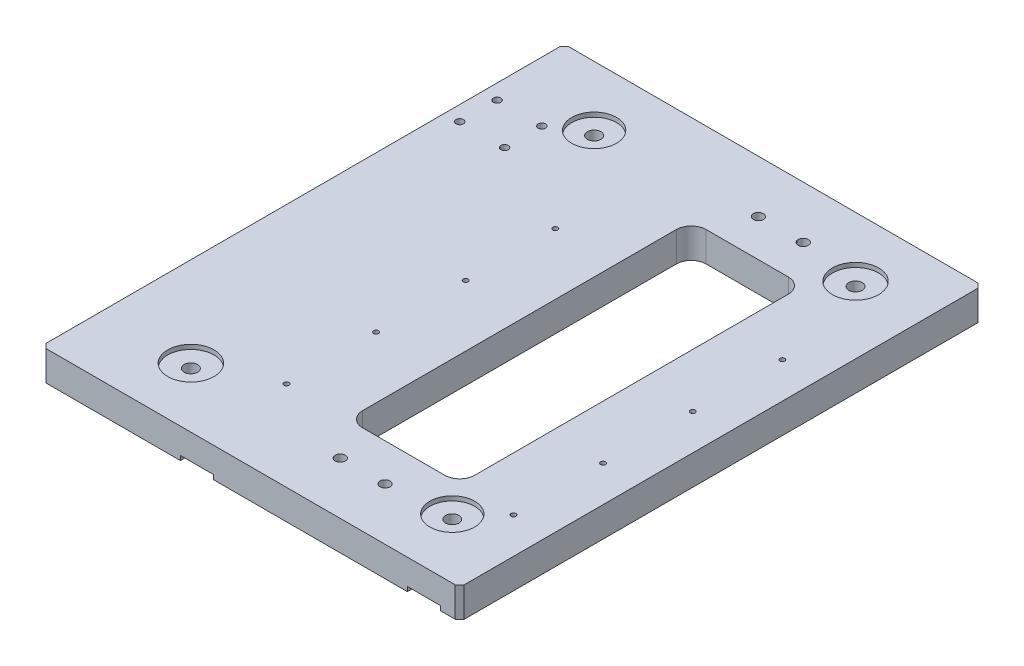
SolidWorks part; units mm, degrees
material "Q235-A"
ref_plane "Front Plane" through (0, 0, 0) normal (0, 0, 1) x (1, 0, 0)
ref_plane "Top Plane" through (0, 0, 0) normal (0, 1, 0) x (1, 0, 0)
ref_plane "Right Plane" through (0, 0, 0) normal (1, 0, 0) x (0, 0, -1)
sketch "Sketch1" plane through (0, 0, 0) normal (0, 0, 1) x (1, 0, 0)
  line L0 (16.7519, 37.3815) -> (146.7519, 37.3815)
  line L1 (-98.2481, 57.3815) -> (181.7519, 57.3815)
  line L2 (-98.2481, 57.3815) -> (-98.2481, 37.3815)
  line L3 (-98.2481, 37.3815) -> (-5.2481, 37.3815)
  line L4 (181.7519, 57.3815) -> (181.7519, 37.3815)
  line L6 (-5.2481, 37.3815) -> (-5.2481, 40.3815)
  line L7 (-5.2481, 40.3815) -> (16.7519, 40.3815)
  line L8 (16.7519, 37.3815) -> (16.7519, 40.3815)
  line L10 (146.7519, 37.3815) -> (146.7519, 40.3815)
  line L11 (146.7519, 40.3815) -> (168.7519, 40.3815)
  line L12 (168.7519, 37.3815) -> (168.7519, 40.3815)
  line L13 (168.7519, 37.3815) -> (181.7519, 37.3815)
  dimension "D1" = 280
  dimension "D2" = 20
  dimension "D3" = 3
  dimension "D4" = 3
  dimension "D5" = 22
  dimension "D6" = 22
  dimension "D7" = 130
  dimension "D8" = 35
extrude "Boss-Extrude1" add sketch "Sketch1" along normal blind 350
chamfer "Chamfer1" distance 3 angle 45 4 edges at (-98.2481, 47.3815, 0) (181.7519, 47.3815, 0) (181.7519, 47.3815, 350) (-98.2481, 47.3815, 350)
sketch "Sketch2" plane through (0, 37.3815, 0) normal (0, -1, 0) x (1, 0, 0)
  line L0 (181.7519, 347) -> (181.7519, 3) construction
  line L1 (46.7519, 290) -> (121.7519, 290)
  line L2 (46.7519, 290) -> (46.7519, 60)
  line L3 (46.7519, 60) -> (121.7519, 60)
  line L4 (121.7519, 290) -> (121.7519, 60)
  line L5 (16.7519, 350) -> (146.7519, 350) construction
  dimension "D1" = 75
  dimension "D2" = 60
  dimension "D3" = 230
  dimension "D4" = 60
extrude "Cut-Extrude1" cut sketch "Sketch2" against normal through all
fillet "Fillet1" radius 10 4 edges at (46.7519, 47.3815, 60) (121.7519, 47.3815, 60) (121.7519, 47.3815, 290) (46.7519, 47.3815, 290)
sketch "Sketch3" plane through (0, 37.3815, 0) normal (0, -1, 0) x (1, 0, 0)
  line L0 (-95.2481, 350) -> (-5.2481, 350) construction
  line L1 (-38.2481, 310) -> (136.7519, 310)
  line L2 (-38.2481, 310) -> (-38.2481, 40)
  line L3 (-38.2481, 40) -> (136.7519, 40)
  line L4 (136.7519, 310) -> (136.7519, 40)
  line L5 (181.7519, 347) -> (181.7519, 3) construction
  dimension "D1" = 175
  dimension "D2" = 270
  dimension "D3" = 40
  dimension "D4" = 45
hole_wizard "Hole1" positions "Sketch4" profile "Sketch5" legacy
sketch "Sketch4" plane through (0, 37.3815, 0) normal (0, -1, 0) x (-1, 0, 0)
  point P0 (38.2481, -310)
  point P3 (-136.7519, -310)
  point P6 (-136.7519, -40)
  point P9 (38.2481, -40)
sketch "Sketch5" plane through (-38.2481, 37.3815, 310) normal (1, 0, 0) x (0, 0, -1)
  line L0 (0, 0) -> (0, 17)
  line L1 (0, 17) -> (4.5, 17)
  line L2 (4.5, 17) -> (4.5, 10.5)
  line L3 (4.5, 10.5) -> (7.5, 10.5)
  line L4 (7.5, 10.5) -> (7.5, 0)
  line L5 (7.5, 0) -> (0, 0)
  line L6 (0, 110) -> (0, -10) construction
  dimension "直径" = 9
  dimension "深度" = 17
  dimension "柱坑直径" = 15
  dimension "柱坑深度" = 10.5
sketch "Sketch6" plane through (0, 40.3815, 0) normal (0, -1, 0) x (1, 0, 0)
  line L0 (-5.2481, 350) -> (-5.2481, 0) construction
  line L1 (-5.2481, 350) -> (16.7519, 350) construction
  circle A0 centre (5.7519, 290) radius 3.6663
  circle A1 centre (157.7519, 290) radius 3.6663
  circle A2 centre (157.7519, 230) radius 3.6663
  circle A3 centre (157.7519, 170) radius 3.6663
  circle A4 centre (157.7519, 110) radius 3.6663
  circle A5 centre (5.7519, 230) radius 3.6663
  circle A6 centre (5.7519, 170) radius 3.6663
  circle A7 centre (5.7519, 110) radius 3.6663
  dimension "D1" = 11
  dimension "D2" = 60
  dimension "D3" = 2
  dimension "D4" = 4
hole_wizard "M4 Tapped Hole1" positions "Sketch7" profile "Sketch8" tap size "M4" standard "GB" end condition through all
sketch "Sketch7" plane through (0, 40.3815, 0) normal (0, -1, 0) x (-1, 0, 0)
  point P0 (-5.7519, -290)
  point P3 (-5.7519, -230)
  point P6 (-5.7519, -170)
  point P9 (-157.7519, -170)
  point P12 (-157.7519, -230)
  point P15 (-157.7519, -290)
  point P18 (-5.7519, -110)
  point P21 (-157.7519, -110)
sketch "Sketch8" plane through (5.7519, 40.3815, 290) normal (1, 0, 0) x (0, 0, -1)
  line L0 (0, 0) -> (0, 17)
  line L1 (0, 17) -> (1.65, 17)
  line L2 (1.65, 17) -> (1.65, 0.375)
  line L3 (1.65, 0.375) -> (2.025, 0)
  line L5 (2.025, 0) -> (0, 0)
  line L6 (-1.65, 0.375) -> (-2.025, 0) construction
  line L11 (0, -6.35) -> (0, 107.95) construction
  dimension "通孔螺纹孔钻头直径" = 3.3
  dimension "通孔螺纹孔钻头深度" = 17
  dimension "近端锥形沉头孔直径" = 4.05
  dimension "近端锥形沉头孔角度" = 90
cosmetic thread "Cosmetic thread 1" parameters "D2"=4
cosmetic thread "Cosmetic thread 2" parameters "D2"=4
cosmetic thread "Cosmetic thread 3" parameters "D2"=4
cosmetic thread "Cosmetic thread 4" parameters "D2"=4
cosmetic thread "Cosmetic thread 5" parameters "D2"=4
cosmetic thread "Cosmetic thread 6" parameters "D2"=4
cosmetic thread "Cosmetic thread 7" parameters "D2"=4
cosmetic thread "Cosmetic thread 8" parameters "D2"=4
sketch "Sketch9" plane through (0, 57.3815, 0) normal (0, 1, 0) x (1, 0, 0)
  line L0 (181.7519, -347) -> (181.7519, -3) construction
  line L1 (136.7519, -310) -> (-38.2481, -310)
  line L2 (136.7519, -310) -> (136.7519, -40)
  line L3 (136.7519, -40) -> (-38.2481, -40)
  line L4 (-38.2481, -310) -> (-38.2481, -40)
  line L5 (178.7519, -350) -> (-95.2481, -350) construction
  line L7 (96.7519, -315) -> (66.7519, -315)
  line L8 (96.7519, -315) -> (96.7519, -35)
  line L9 (96.7519, -35) -> (66.7519, -35)
  line L10 (66.7519, -315) -> (66.7519, -35)
  line L11 (-58.2481, -80) -> (-88.2481, -80)
  line L12 (-58.2481, -80) -> (-58.2481, -55)
  line L13 (-58.2481, -55) -> (-88.2481, -55)
  line L14 (-88.2481, -80) -> (-88.2481, -55)
  point P12 (96.7519, -175)
  point P13 (136.7519, -175)
  dimension "D1" = 270
  dimension "D2" = 175
  dimension "D3" = 45
  dimension "D4" = 40
  dimension "D5" = 280
  dimension "D6" = 30
  dimension "D7" = 85
  dimension "D8" = 0
  dimension "D9" = 30
  dimension "D10" = 25
  dimension "D11" = 240
  dimension "D12" = 270
hole_wizard "Hole2" positions "Sketch10" profile "Sketch11" legacy
sketch "Sketch10" plane through (0, 57.3815, 0) normal (0, 1, 0) x (1, 0, 0)
  point P0 (-38.2481, -310)
  point P3 (136.7519, -40)
sketch "Sketch11" plane through (-38.2481, 57.3815, 310) normal (1, 0, 0) x (0, 0, 1)
  line L0 (0, 0) -> (0, 3)
  line L1 (0, 3) -> (15.5, 3)
  line L2 (15.5, 3) -> (15.5, 0)
  line L3 (15.5, 0) -> (0, 0)
  line L4 (0, 110) -> (0, -10) construction
  dimension "直径" = 31
  dimension "深度" = 3
hole_wizard "Hole3" positions "Sketch12" profile "Sketch13" legacy
sketch "Sketch12" plane through (0, 57.3815, 0) normal (0, 1, 0) x (1, 0, 0)
  point P0 (-38.2481, -40)
  point P3 (136.7519, -310)
sketch "Sketch13" plane through (-38.2481, 57.3815, 40) normal (1, 0, 0) x (0, 0, 1)
  line L0 (0, 0) -> (0, 3)
  line L1 (0, 3) -> (15, 3)
  line L2 (15, 3) -> (15, 0)
  line L3 (15, 0) -> (0, 0)
  line L4 (0, 110) -> (0, -10) construction
  dimension "直径" = 30
  dimension "深度" = 3
hole_wizard "M8 Tapped Hole1" positions "Sketch14" profile "Sketch15" tap size "M8" standard "GB" end condition through all
sketch "Sketch14" plane through (0, 57.3815, 0) normal (0, 1, 0) x (1, 0, 0)
  point P0 (96.7519, -315)
  point P3 (66.7519, -315)
  point P6 (96.7519, -35)
  point P9 (66.7519, -35)
sketch "Sketch15" plane through (96.7519, 57.3815, 315) normal (1, 0, 0) x (0, 0, 1)
  line L0 (0, 0) -> (0, 20)
  line L1 (0, 20) -> (3.4, 20)
  line L2 (3.4, 20) -> (3.4, 0)
  line L5 (3.4, 0) -> (0, 0)
  line L11 (0, -6.35) -> (0, 107.95) construction
  dimension "通孔螺纹孔钻头直径" = 6.8
  dimension "通孔螺纹孔钻头深度" = 20
cosmetic thread "Cosmetic thread 9" parameters "D2"=8
cosmetic thread "Cosmetic thread 10" parameters "D2"=8
cosmetic thread "Cosmetic thread 11" parameters "D2"=8
cosmetic thread "Cosmetic thread 12" parameters "D2"=8
hole_wizard "M6 Tapped Hole2" positions "Sketch18" profile "Sketch19" tap size "M6" standard "GB" end condition through all
sketch "Sketch18" plane through (0, 57.3815, 0) normal (0, 1, 0) x (1, 0, 0)
  point P0 (-58.2481, -80)
  point P3 (-58.2481, -55)
  point P6 (-88.2481, -55)
  point P9 (-88.2481, -80)
sketch "Sketch19" plane through (-58.2481, 57.3815, 80) normal (1, 0, 0) x (0, 0, 1)
  line L0 (0, 0) -> (0, 20)
  line L1 (0, 20) -> (2.5, 20)
  line L2 (2.5, 20) -> (2.5, 0)
  line L5 (2.5, 0) -> (0, 0)
  line L11 (0, -6.35) -> (0, 107.95) construction
  dimension "通孔螺纹孔钻头直径" = 5
  dimension "通孔螺纹孔钻头深度" = 20
cosmetic thread "Cosmetic thread 17" parameters "D2"=6
cosmetic thread "Cosmetic thread 18" parameters "D2"=6
cosmetic thread "Cosmetic thread 19" parameters "D2"=6
cosmetic thread "Cosmetic thread 20" parameters "D2"=6
